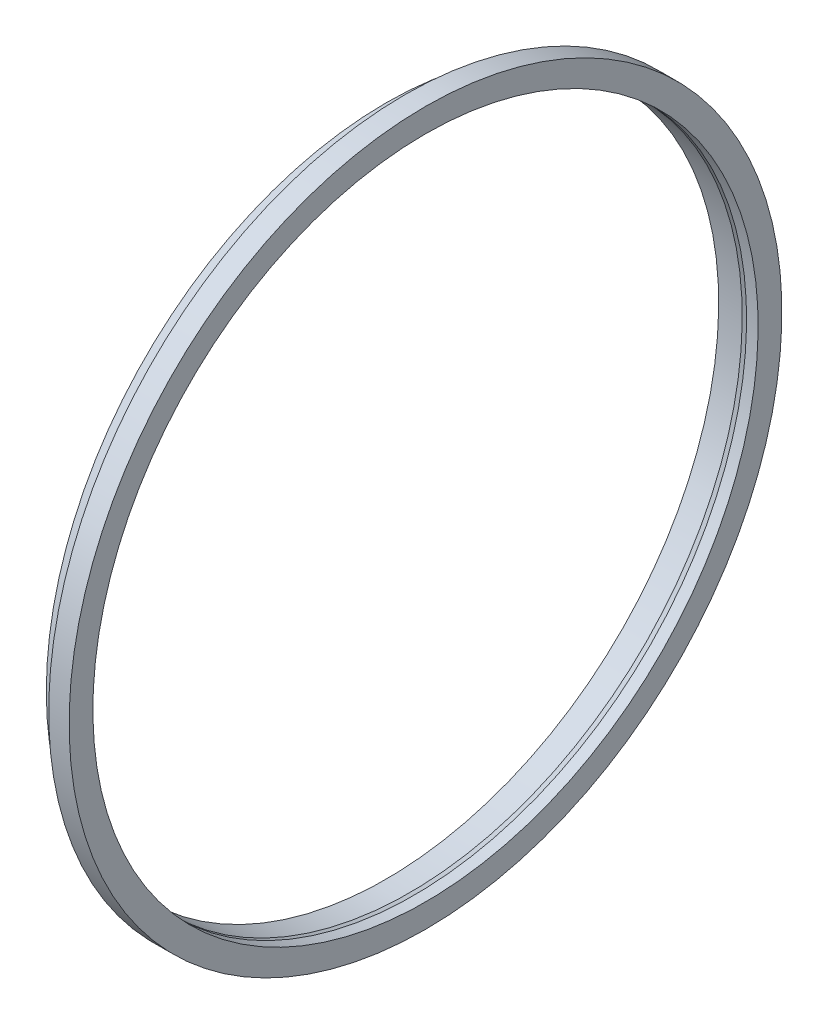
SolidWorks part; units mm, degrees
ref_plane "Front Plane" through (0, 0, 0) normal (0, 0, 1) x (1, 0, 0)
ref_plane "Top Plane" through (0, 0, 0) normal (0, 1, 0) x (1, 0, 0)
ref_plane "Right Plane" through (0, 0, 0) normal (1, 0, 0) x (0, 0, -1)
sketch "Sketch1" plane through (0, 0, 0) normal (0, 0, 1) x (1, 0, 0)
  line L0 (0, 0) -> (-70, 0)
  line L1 (-70, 70) -> (-70, 71.5)
  line L4 (-66, 75) -> (-61.7, 75)
  line L5 (-61.7, 75) -> (-61.7, 70)
  line L6 (-61.7, 70) -> (-64.1279, 70)
  line L7 (-66, 75) -> (-66, 72.65)
  line L8 (-66, 72.65) -> (-70, 71.5)
  line L9 (-65.0501, 70) -> (-64.1279, 70.5469)
  line L10 (-64.1279, 70.5469) -> (-64.1279, 70)
  line L11 (-65.0501, 70) -> (-70, 70)
  point P10 (-62.9139, 70)
  dimension "D1" = 70
  dimension "D2" = 5
  dimension "D3" = 4.3
  dimension "D4" = 4
  dimension "D5" = 2.35
  dimension "D6" = 1.5
  dimension "D7" = 70
revolve "Revolve1" add sketch "Sketch1" angle 360 about L0
